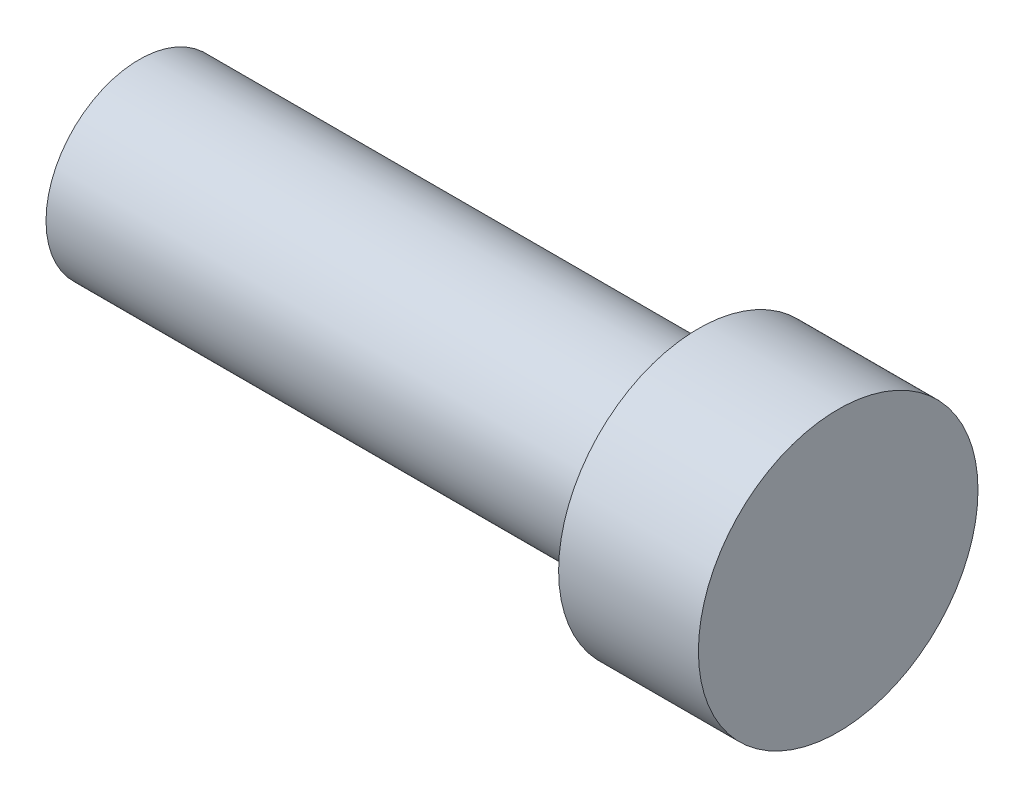
SolidWorks part; units mm, degrees
material "1023 碳钢板 (SS)"
ref_plane "Front Plane" through (0, 0, 0) normal (0, 0, 1) x (1, 0, 0)
ref_plane "Top Plane" through (0, 0, 0) normal (0, 1, 0) x (1, 0, 0)
ref_plane "Right Plane" through (0, 0, 0) normal (1, 0, 0) x (0, 0, -1)
sketch "Sketch1" plane through (0, 0, 0) normal (0, 0, 1) x (1, 0, 0)
  line L0 (1184.079, 97.6011) -> (1196.079, 97.6011)
  line L1 (1184.079, 97.6011) -> (1184.079, 95.6011)
  line L2 (1196.079, 97.6011) -> (1196.079, 95.6011)
  line L3 (1196.079, 97.6011) -> (1196.079, 98.6011)
  line L4 (1196.079, 98.6011) -> (1199.079, 98.6011)
  line L5 (1199.079, 95.6011) -> (1199.079, 98.6011)
  line L6 (1184.079, 95.6011) -> (1199.079, 95.6011)
revolve "Revolve1" add sketch "Sketch1" angle 360 about L6
